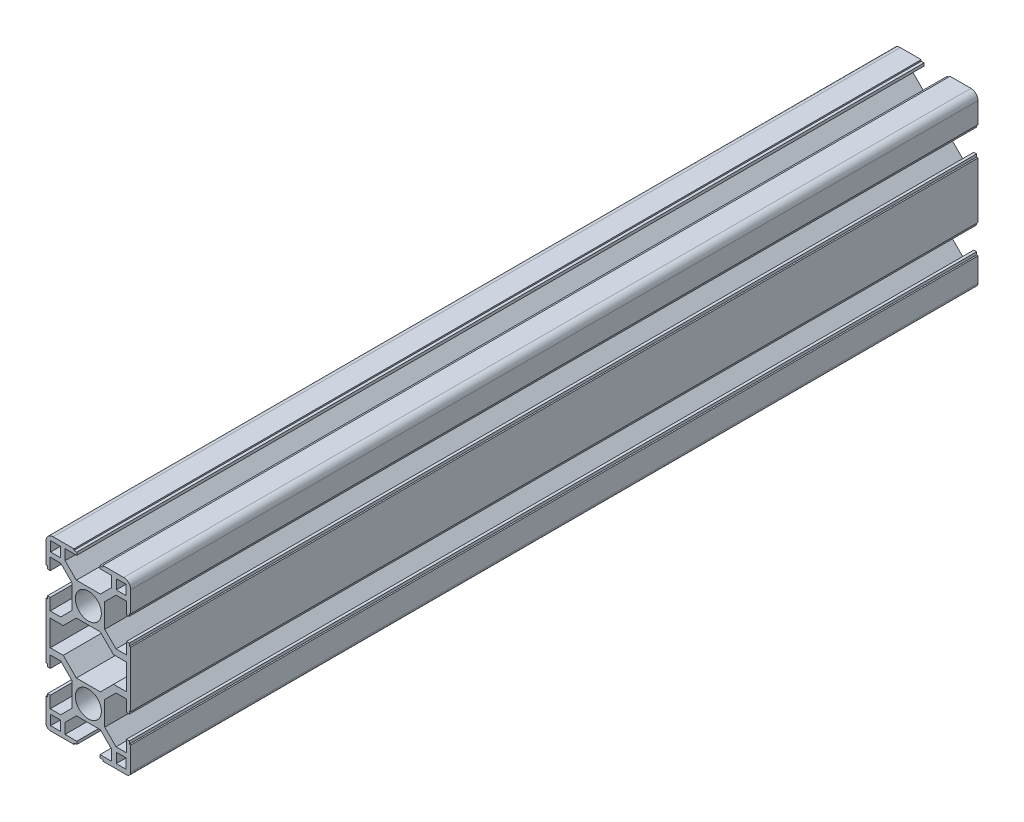
from build123d import *

# Parameters (mm, degrees)
SKETCH1_R                 = 4.6
SKETCH1_W                 = 3.5
SKETCH1_H                 = 3.5
F_30_X_60L_X_R2_5_1_DEPTH = 300


with BuildPart() as part:
    # Sketch1 → 铝型材 30 X 60L X R2.5(1) (new body)
    with BuildSketch(Plane(origin=(0, 0, 0), x_dir=(-1, 0, 0), z_dir=(0, 0, -1))):
        with BuildLine():
            Line((-5.1, 15), (-5.1, 14.5))
            Line((-5.1, 14.5), (-4.1, 14.5))
            Line((-4.1, 14.5), (-4.1, 13.5))
            Line((-4.1, 13.5), (-8.25, 13.5))
            Line((-8.25, 13.5), (-8.25, 9.8))
            Line((-8.25, 9.8), (-4.25, 5.8))
            Line((-4.25, 5.8), (4.25, 5.8))
            Line((4.25, 5.8), (8.25, 9.8))
            Line((8.25, 9.8), (8.25, 13.5))
            Line((8.25, 13.5), (4.1, 13.5))
            Line((4.1, 13.5), (4.1, 14.5))
            Line((4.1, 14.5), (5.1, 14.5))
            Line((5.1, 14.5), (5.1, 15))
            Line((5.1, 15), (12.5, 15))
            ThreePointArc((12.5, 15), (14.267766953, 14.267766953), (15, 12.5))
            Line((15, 12.5), (15, 5.1))
            Line((15, 5.1), (14.5, 5.1))
            Line((14.5, 5.1), (14.5, 4.1))
            Line((14.5, 4.1), (13.5, 4.1))
            Line((13.5, 4.1), (13.5, 8.25))
            Line((13.5, 8.25), (9.8, 8.25))
            Line((9.8, 8.25), (5.8, 4.25))
            Line((5.8, 4.25), (5.8, -4.25))
            Line((5.8, -4.25), (9.8, -8.25))
            Line((9.8, -8.25), (13.5, -8.25))
            Line((13.5, -8.25), (13.5, -4.1))
            Line((13.5, -4.1), (14.5, -4.1))
            Line((14.5, -4.1), (14.5, -5.1))
            Line((14.5, -5.1), (15, -5.1))
            Line((15, -5.1), (15, -24.9))
            Line((15, -24.9), (14.5, -24.9))
            Line((14.5, -24.9), (14.5, -25.9))
            Line((14.5, -25.9), (13.5, -25.9))
            Line((13.5, -25.9), (13.5, -21.75))
            Line((13.5, -21.75), (9.8, -21.75))
            Line((9.8, -21.75), (5.8, -25.75))
            Line((5.8, -25.75), (5.8, -34.25))
            Line((5.8, -34.25), (9.8, -38.25))
            Line((9.8, -38.25), (13.5, -38.25))
            Line((13.5, -38.25), (13.5, -34.1))
            Line((13.5, -34.1), (14.5, -34.1))
            Line((14.5, -34.1), (14.5, -35.1))
            Line((14.5, -35.1), (15, -35.1))
            Line((15, -35.1), (15, -43.5))
            ThreePointArc((15, -43.5), (14.560660172, -44.560660172), (13.5, -45))
            Line((13.5, -45), (5.1, -45))
            Line((5.1, -45), (5.1, -44.5))
            Line((5.1, -44.5), (4.1, -44.5))
            Line((4.1, -44.5), (4.1, -43.5))
            Line((4.1, -43.5), (8.25, -43.5))
            Line((8.25, -43.5), (8.25, -39.8))
            Line((8.25, -39.8), (4.25, -35.8))
            Line((4.25, -35.8), (-4.25, -35.8))
            Line((-4.25, -35.8), (-8.25, -39.8))
            Line((-8.25, -39.8), (-8.25, -43.5))
            Line((-8.25, -43.5), (-4.1, -43.5))
            Line((-4.1, -43.5), (-4.1, -44.5))
            Line((-4.1, -44.5), (-5.1, -44.5))
            Line((-5.1, -44.5), (-5.1, -45))
            Line((-5.1, -45), (-13.5, -45))
            ThreePointArc((-13.5, -45), (-14.560660172, -44.560660172), (-15, -43.5))
            Line((-15, -43.5), (-15, -35.1))
            Line((-15, -35.1), (-14.5, -35.1))
            Line((-14.5, -35.1), (-14.5, -34.1))
            Line((-14.5, -34.1), (-13.5, -34.1))
            Line((-13.5, -34.1), (-13.5, -38.25))
            Line((-13.5, -38.25), (-9.8, -38.25))
            Line((-9.8, -38.25), (-5.8, -34.25))
            Line((-5.8, -34.25), (-5.8, -25.75))
            Line((-5.8, -25.75), (-9.8, -21.75))
            Line((-9.8, -21.75), (-13.5, -21.75))
            Line((-13.5, -21.75), (-13.5, -25.9))
            Line((-13.5, -25.9), (-14.5, -25.9))
            Line((-14.5, -25.9), (-14.5, -24.9))
            Line((-14.5, -24.9), (-15, -24.9))
            Line((-15, -24.9), (-15, -5.1))
            Line((-15, -5.1), (-14.5, -5.1))
            Line((-14.5, -5.1), (-14.5, -4.1))
            Line((-14.5, -4.1), (-13.5, -4.1))
            Line((-13.5, -4.1), (-13.5, -8.25))
            Line((-13.5, -8.25), (-9.8, -8.25))
            Line((-9.8, -8.25), (-5.8, -4.25))
            Line((-5.8, -4.25), (-5.8, 4.25))
            Line((-5.8, 4.25), (-9.8, 8.25))
            Line((-9.8, 8.25), (-13.5, 8.25))
            Line((-13.5, 8.25), (-13.5, 4.1))
            Line((-13.5, 4.1), (-14.5, 4.1))
            Line((-14.5, 4.1), (-14.5, 5.1))
            Line((-14.5, 5.1), (-15, 5.1))
            Line((-15, 5.1), (-15, 12.5))
            ThreePointArc((-15, 12.5), (-14.267766953, 14.267766953), (-12.5, 15))
            Line((-12.5, 15), (-5.1, 15))
        make_face()
        Circle(SKETCH1_R, mode=Mode.SUBTRACT)
        with Locations((0, -30)):
            Circle(SKETCH1_R, mode=Mode.SUBTRACT)
        Polygon((8.9, -10.45), (4.25, -5.8), (-4.25, -5.8), (-8.9, -10.45), (-13.5, -10.45), (-13.5, -19.55), (-8.9, -19.55), (-4.25, -24.2), (4.25, -24.2), (8.9, -19.55), (13.5, -19.55), (13.5, -10.45), align=None, mode=Mode.SUBTRACT)
        with Locations((-11.625, 11.625)):
            Rectangle(SKETCH1_W, SKETCH1_H, mode=Mode.SUBTRACT)
        with Locations((11.625, 11.625)):
            Rectangle(SKETCH1_W, SKETCH1_H, mode=Mode.SUBTRACT)
        with Locations((-11.625, -41.625)):
            Rectangle(SKETCH1_W, SKETCH1_H, mode=Mode.SUBTRACT)
        with Locations((11.625, -41.625)):
            Rectangle(SKETCH1_W, SKETCH1_H, mode=Mode.SUBTRACT)
    extrude(amount=F_30_X_60L_X_R2_5_1_DEPTH)


solid = part.part
